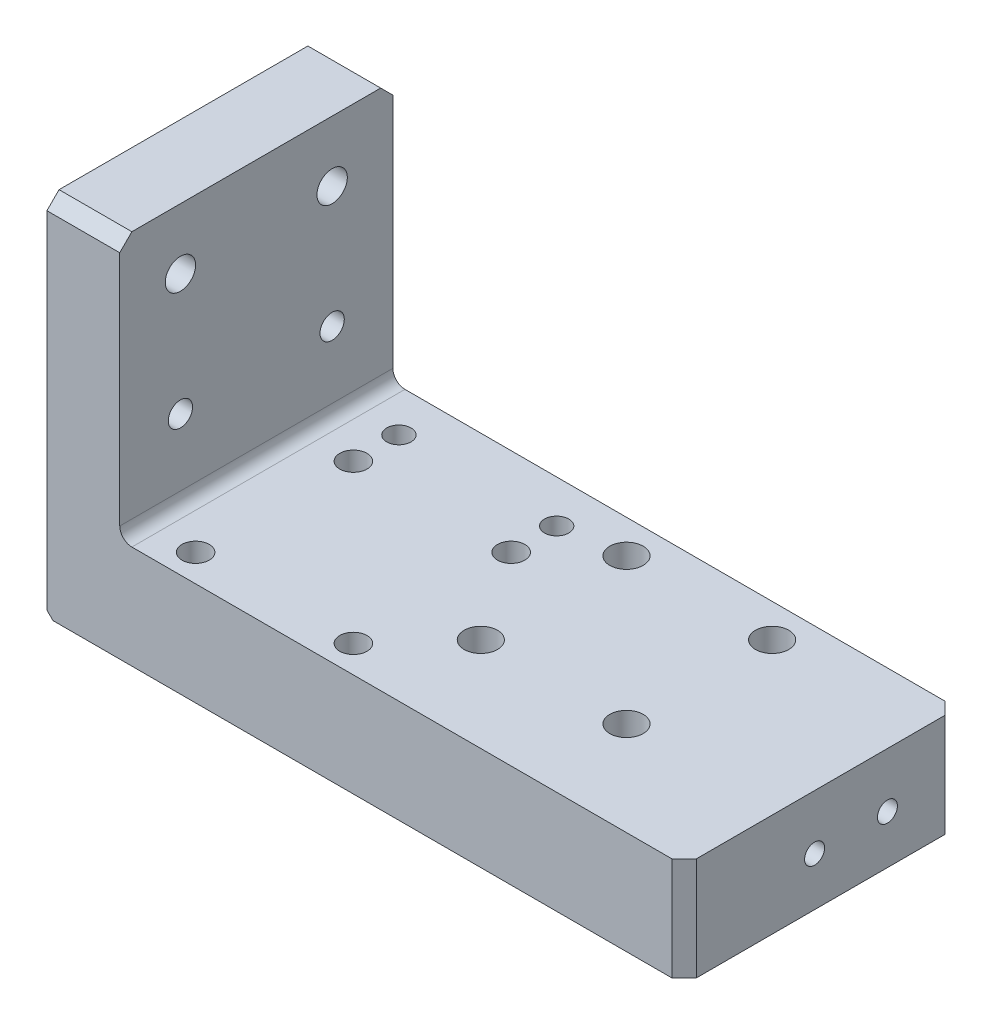
from build123d import *

# Parameters (mm, degrees)
BOSS_EXTRUDE1_DEPTH                                  = 22.5
HOLE_SIZE_PER_SOCKET_HEAD_CAP_SCREW_TYPE_D           = 5.5
HOLE_SIZE_PER_SOCKET_HEAD_CAP_SCREW_TYPE_CBORE_D     = 10
HOLE_SIZE_PER_SOCKET_HEAD_CAP_SCREW_TYPE_CBORE_DEPTH = 5.7
F_4_5_4_5_DIAMETER_HOLE1_D                           = 4.5
M4_TAPPED_HOLE1_D                                    = 3.3
M4_TAPPED_HOLE1_DEPTH                                = 10.1
M4_TAPPED_HOLE1_TIP                                  = 0.991420021
M6_TAPPED_HOLE1_D                                    = 5
M6_TAPPED_HOLE1_DEPTH                                = 15
M6_TAPPED_HOLE1_TIP                                  = 1.502151548
F_4_0_4_DIAMETER_HOLE1_D                             = 4
F_4_0_4_DIAMETER_HOLE1_DEPTH                         = 15
F_4_0_4_DIAMETER_HOLE1_TIP                           = 1.201721238
F_4_0_4_DIAMETER_HOLE2_D                             = 4
F_4_0_4_DIAMETER_HOLE2_DEPTH                         = 17
F_4_0_4_DIAMETER_HOLE2_TIP                           = 1.201721238
CHAMFER1_SIZE                                        = 2
CHAMFER2_SIZE                                        = 1
FILLET1_R                                            = 2


with BuildPart() as part:
    # Sketch1 → Boss-Extrude1 (new, symmetric)
    with BuildSketch(Plane.XY):
        Polygon((0, 0), (0, 60), (12, 60), (12, 17), (105, 17), (105, 0), align=None)
    extrude(amount=BOSS_EXTRUDE1_DEPTH, both=True)

    # Hole size per socket head cap screw type 1 (through all)
    with Locations(Plane(origin=(0, 0, 0), x_dir=(-1, 0, 0), z_dir=(0, -1, 0))):
        with Locations((-80, -7), (-56, -7), (-56, 17), (-80, 17)):
            CounterBoreHole(HOLE_SIZE_PER_SOCKET_HEAD_CAP_SCREW_TYPE_D / 2, HOLE_SIZE_PER_SOCKET_HEAD_CAP_SCREW_TYPE_CBORE_D / 2, HOLE_SIZE_PER_SOCKET_HEAD_CAP_SCREW_TYPE_CBORE_DEPTH)

    # Ø4.5 (4.5) Diameter Hole1 (through all)
    with Locations(Plane(origin=(0, 17, 0), x_dir=(1, 0, 0), z_dir=(0, 1, 0))):
        with Locations((20, 8), (46, 8), (20, -18), (46, -18)):
            Hole(F_4_5_4_5_DIAMETER_HOLE1_D / 2)

    # M4 Tapped Hole1
    with Locations(Plane(origin=(105, 0, 0), x_dir=(0, 0, -1), z_dir=(1, 0, 0))):
        with Locations((-1, 8), (11, 8)):
            Hole(M4_TAPPED_HOLE1_D / 2, depth=M4_TAPPED_HOLE1_DEPTH)
            with Locations((0, 0, -(M4_TAPPED_HOLE1_DEPTH + M4_TAPPED_HOLE1_TIP / 2))):  # 118° drill point
                Cone(0, M4_TAPPED_HOLE1_D / 2, M4_TAPPED_HOLE1_TIP, mode=Mode.SUBTRACT)

    # M6 Tapped Hole1
    with Locations(Plane.ZY):
        with Locations((-12.5, 50), (12.5, 50), (-12.5, 10), (12.5, 10)):
            Hole(M6_TAPPED_HOLE1_D / 2, depth=M6_TAPPED_HOLE1_DEPTH)
            with Locations((0, 0, -(M6_TAPPED_HOLE1_DEPTH + M6_TAPPED_HOLE1_TIP / 2))):  # 118° drill point
                Cone(0, M6_TAPPED_HOLE1_D / 2, M6_TAPPED_HOLE1_TIP, mode=Mode.SUBTRACT)

    # Ø4.0 (4) Diameter Hole1
    with Locations(Plane.ZY):
        with Locations((-12.5, 30), (12.5, 30)):
            Hole(F_4_0_4_DIAMETER_HOLE1_D / 2, depth=F_4_0_4_DIAMETER_HOLE1_DEPTH)
            with Locations((0, 0, -(F_4_0_4_DIAMETER_HOLE1_DEPTH + F_4_0_4_DIAMETER_HOLE1_TIP / 2))):  # 118° drill point
                Cone(0, F_4_0_4_DIAMETER_HOLE1_D / 2, F_4_0_4_DIAMETER_HOLE1_TIP, mode=Mode.SUBTRACT)

    # Ø4.0 (4) Diameter Hole2
    with Locations(Plane(origin=(0, 0, 0), x_dir=(-1, 0, 0), z_dir=(0, -1, 0))):
        with Locations((-20, 15.5), (-46, 15.5)):
            Hole(F_4_0_4_DIAMETER_HOLE2_D / 2, depth=F_4_0_4_DIAMETER_HOLE2_DEPTH)
            with Locations((0, 0, -(F_4_0_4_DIAMETER_HOLE2_DEPTH + F_4_0_4_DIAMETER_HOLE2_TIP / 2))):  # 118° drill point
                Cone(0, F_4_0_4_DIAMETER_HOLE2_D / 2, F_4_0_4_DIAMETER_HOLE2_TIP, mode=Mode.SUBTRACT)

    # Chamfer1
    chamfer1_edges = [part.edges().sort_by_distance(p)[0] for p in [
        (6, 60, 22.5),
        (6, 60, -22.5),
        (105, 8.5, 22.5),
        (105, 8.5, -22.5),
    ]]
    chamfer(chamfer1_edges, length=CHAMFER1_SIZE)

    # Chamfer2
    chamfer2_edges = [part.edges().sort_by_distance(p)[0] for p in [
        (0, 0, 0),
    ]]
    chamfer(chamfer2_edges, length=CHAMFER2_SIZE)

    # Fillet1
    fillet1_edges = [part.edges().sort_by_distance(p)[0] for p in [
        (12, 17, 0),
    ]]
    fillet(fillet1_edges, radius=FILLET1_R)


solid = part.part
